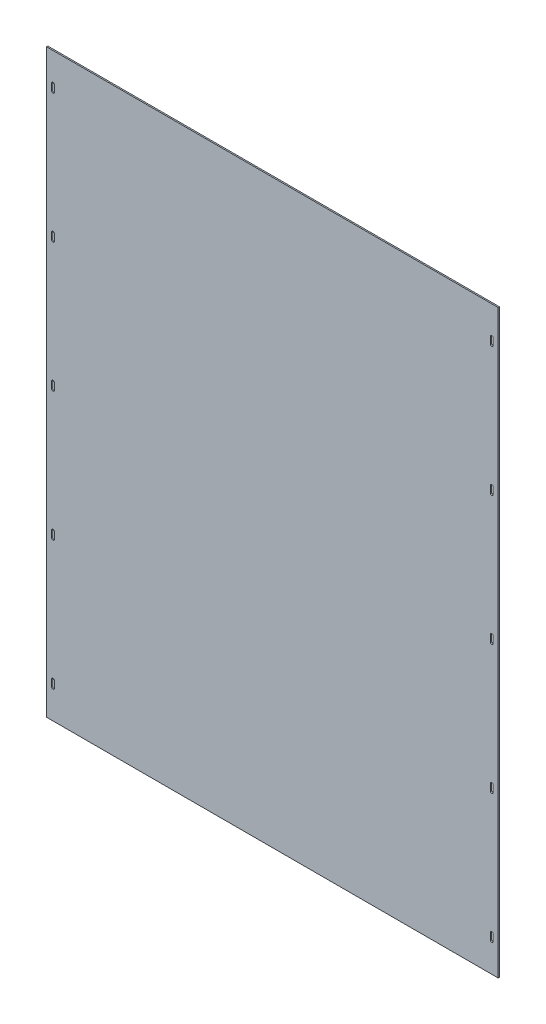
SolidWorks part; units mm, degrees
material "普通碳钢"
ref_plane "前视基准面" through (0, 0, 0) normal (0, 0, 1) x (1, 0, 0)
ref_plane "上视基准面" through (0, 0, 0) normal (0, 1, 0) x (1, 0, 0)
ref_plane "右视基准面" through (0, 0, 0) normal (1, 0, 0) x (0, 0, -1)
sketch "草图1" plane through (0, 0, 0) normal (0, 0, 1) x (1, 0, 0)
  line L1 (-350, 450) -> (350, 450)
  line L2 (-350, 450) -> (-350, -450)
  line L3 (-350, -450) -> (350, -450)
  line L4 (350, 450) -> (350, -450)
  line L5 (0, -450) -> (0, 450) construction
  line L6 (-350, 0) -> (350, 0) construction
  point P0 (0, 0)
  dimension "D1" = 700
  dimension "D2" = 900
extrude "凸台-拉伸1" add sketch "草图1" along normal blind 2
sketch "草图2" plane through (0, 0, 2) normal (0, 0, 1) x (1, 0, 0)
  line L0 (0, 450) -> (0, -450) construction
  line L1 (350, 450) -> (-350, 450) construction
  line L2 (-350, -450) -> (350, -450) construction
  line L3 (-340, 405) -> (-340, 395) construction
  line L4 (-340, -400) -> (340, -400) construction
  line L5 (-340, -400) -> (-340, 400) construction
  line L6 (-340, 400) -> (340, 400) construction
  line L7 (340, -400) -> (340, 400) construction
  line L8 (0, 400) -> (0, -400) construction
  line L9 (-340, 0) -> (340, 0) construction
  line L10 (-337.75, 405) -> (-337.75, 395)
  line L11 (-342.25, 405) -> (-342.25, 395)
  line L12 (340, 405) -> (340, 395) construction
  line L13 (337.75, 405) -> (337.75, 395)
  line L14 (342.25, 405) -> (342.25, 395)
  line L15 (-340, 195) -> (-340, 205) construction
  line L16 (-342.25, 195) -> (-342.25, 205)
  line L17 (-337.75, 195) -> (-337.75, 205)
  line L18 (-340, -5) -> (-340, 5) construction
  line L19 (-342.25, -5) -> (-342.25, 5)
  line L20 (-337.75, -5) -> (-337.75, 5)
  line L21 (340, 195) -> (340, 205) construction
  line L22 (342.25, 195) -> (342.25, 205)
  line L23 (337.75, 195) -> (337.75, 205)
  line L24 (340, -5) -> (340, 5) construction
  line L25 (342.25, -5) -> (342.25, 5)
  line L26 (337.75, -5) -> (337.75, 5)
  line L27 (-340, 605) -> (-340, 595) construction
  line L28 (-342.25, 605) -> (-342.25, 595)
  line L29 (-337.75, 605) -> (-337.75, 595)
  line L30 (340, 605) -> (340, 595) construction
  line L31 (342.25, 605) -> (342.25, 595)
  line L32 (337.75, 605) -> (337.75, 595)
  line L33 (-340, -400) -> (340, -400) construction
  line L34 (340, -195) -> (340, -205) construction
  line L35 (342.25, -195) -> (342.25, -205)
  line L36 (337.75, -195) -> (337.75, -205)
  line L37 (-340, -195) -> (-340, -205) construction
  line L38 (-342.25, -195) -> (-342.25, -205)
  line L39 (-337.75, -195) -> (-337.75, -205)
  line L40 (340, -405) -> (340, -395) construction
  line L41 (337.75, -405) -> (337.75, -395)
  line L42 (342.25, -405) -> (342.25, -395)
  line L43 (-340, -405) -> (-340, -395) construction
  line L44 (-337.75, -405) -> (-337.75, -395)
  line L45 (-342.25, -405) -> (-342.25, -395)
  arc A0 (-337.75, 405) -> (-342.25, 405) centre (-340, 405) ccw
  arc A1 (-342.25, 395) -> (-337.75, 395) centre (-340, 395) ccw
  arc A2 (337.75, 405) -> (342.25, 405) centre (340, 405) cw
  arc A3 (342.25, 395) -> (337.75, 395) centre (340, 395) cw
  arc A4 (-342.25, 195) -> (-337.75, 195) centre (-340, 195) ccw
  arc A5 (-337.75, 205) -> (-342.25, 205) centre (-340, 205) ccw
  arc A6 (-342.25, -5) -> (-337.75, -5) centre (-340, -5) ccw
  arc A7 (-337.75, 5) -> (-342.25, 5) centre (-340, 5) ccw
  arc A8 (342.25, 195) -> (337.75, 195) centre (340, 195) cw
  arc A9 (337.75, 205) -> (342.25, 205) centre (340, 205) cw
  arc A10 (342.25, -5) -> (337.75, -5) centre (340, -5) cw
  arc A11 (337.75, 5) -> (342.25, 5) centre (340, 5) cw
  arc A12 (-342.25, 605) -> (-337.75, 605) centre (-340, 605) cw
  arc A13 (-337.75, 595) -> (-342.25, 595) centre (-340, 595) cw
  arc A14 (342.25, 605) -> (337.75, 605) centre (340, 605) ccw
  arc A15 (337.75, 595) -> (342.25, 595) centre (340, 595) ccw
  arc A16 (342.25, -195) -> (337.75, -195) centre (340, -195) ccw
  arc A17 (337.75, -205) -> (342.25, -205) centre (340, -205) ccw
  arc A18 (-342.25, -195) -> (-337.75, -195) centre (-340, -195) cw
  arc A19 (-337.75, -205) -> (-342.25, -205) centre (-340, -205) cw
  arc A20 (337.75, -405) -> (342.25, -405) centre (340, -405) ccw
  arc A21 (342.25, -395) -> (337.75, -395) centre (340, -395) ccw
  arc A22 (-337.75, -405) -> (-342.25, -405) centre (-340, -405) cw
  arc A23 (-342.25, -395) -> (-337.75, -395) centre (-340, -395) cw
  point P6 (0, 0)
  point P12 (-340, 400)
  point P19 (340, 400)
  point P26 (-340, 200)
  point P32 (-340, 0)
  point P40 (340, 200)
  point P47 (340, 0)
  point P54 (-340, 600)
  point P61 (340, 600)
  point P68 (340, -200)
  point P75 (-340, -200)
  point P82 (340, -400)
  point P89 (-340, -400)
  dimension "D1" = 680
  dimension "D2" = 800
  dimension "D3" = 4.5
  dimension "D4" = 10
  dimension "D5" = 10
  dimension "D6" = 10
  dimension "D7" = 4.5
  dimension "D8" = 4.5
  dimension "D9" = 200
extrude "切除-拉伸1" cut sketch "草图2" against normal blind 10
